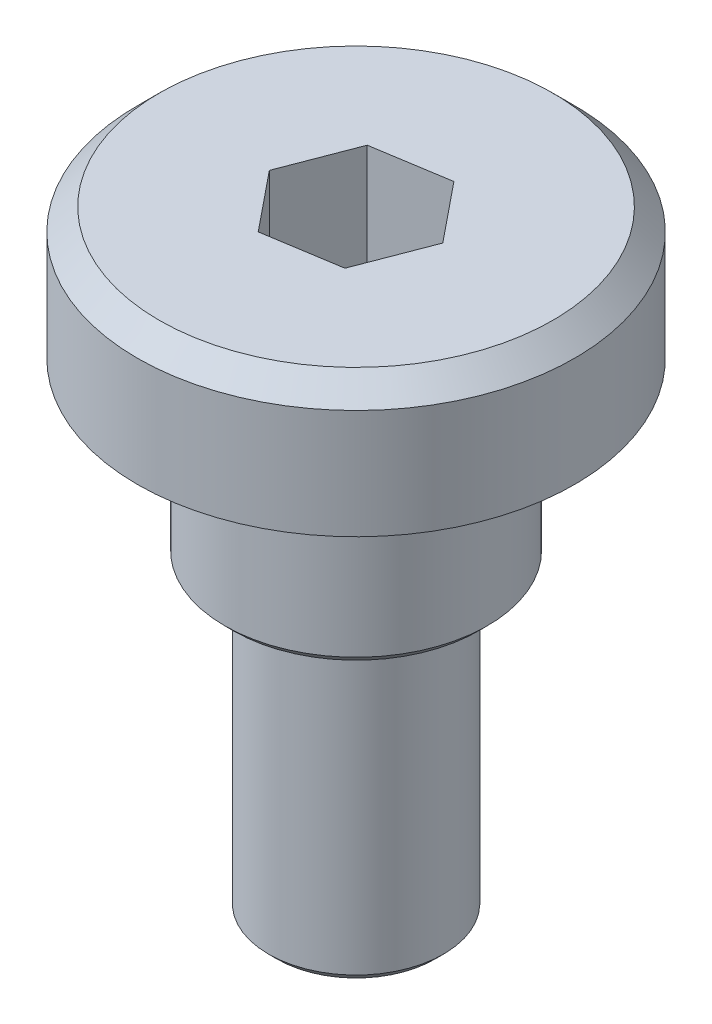
from build123d import *

# Parameters (mm, degrees)
SKETCH_1_R          = 2
EXTRUDE_1_DEPTH     = 7
SKETCH_2_R          = 3
EXTRUDE_2_DEPTH     = 4
SKETCH_3_R          = 5
EXTRUDE_3_DEPTH     = 3
CHAMFER_1_SIZE      = 0.5
CHAMFER_2_SIZE      = 0.2
CHAMFER_3_SIZE      = 0.2
CUT_EXTRUDE_1_DEPTH = 3


with BuildPart() as part:
    # 草图1 → 凸台-拉伸1 (new body)
    with BuildSketch(Plane(origin=(0, 0, 0), x_dir=(1, 0, 0), z_dir=(0, 1, 0))):
        with Locations(Location((0, 0, 0), (0, 0, 270))):
            Circle(SKETCH_1_R)
    extrude(amount=EXTRUDE_1_DEPTH)

    # 草图2 → 凸台-拉伸2 (add)
    with BuildSketch(Plane(origin=(0, 7, 0), x_dir=(1, 0, 0), z_dir=(0, 1, 0))):
        with Locations(Location((0, 0, 0), (0, 0, 270))):
            Circle(SKETCH_2_R)
    extrude(amount=EXTRUDE_2_DEPTH)

    # 草图3 → 凸台-拉伸3 (add)
    with BuildSketch(Plane(origin=(0, 11, 0), x_dir=(1, 0, 0), z_dir=(0, 1, 0))):
        with Locations(Location((0, 0, 0), (0, 0, 270))):
            Circle(SKETCH_3_R)
    extrude(amount=EXTRUDE_3_DEPTH)

    # 倒角1
    chamfer_1_edges = [part.edges().sort_by_distance(p)[0] for p in [
        (0, 14, -5),
    ]]
    chamfer(chamfer_1_edges, length=CHAMFER_1_SIZE)

    # 倒角2
    chamfer_2_edges = [part.edges().sort_by_distance(p)[0] for p in [
        (0, 7, -3),
    ]]
    chamfer(chamfer_2_edges, length=CHAMFER_2_SIZE)

    # 倒角3
    chamfer_3_edges = [part.edges().sort_by_distance(p)[0] for p in [
        (0, 0, -2),
    ]]
    chamfer(chamfer_3_edges, length=CHAMFER_3_SIZE)

    # 草图4 → 切除-拉伸1 (cut)
    with BuildSketch(Plane(origin=(0, 14, 0), x_dir=(1, 0, 0), z_dir=(0, 1, 0))):
        Polygon((1.090848991, -1.345380422), (1.710558118, 0.272012727), (0.619709128, 1.617393149), (-1.090848991, 1.345380422), (-1.710558118, -0.272012727), (-0.619709128, -1.617393149), align=None)
    extrude(amount=-CUT_EXTRUDE_1_DEPTH, mode=Mode.SUBTRACT)


solid = part.part
